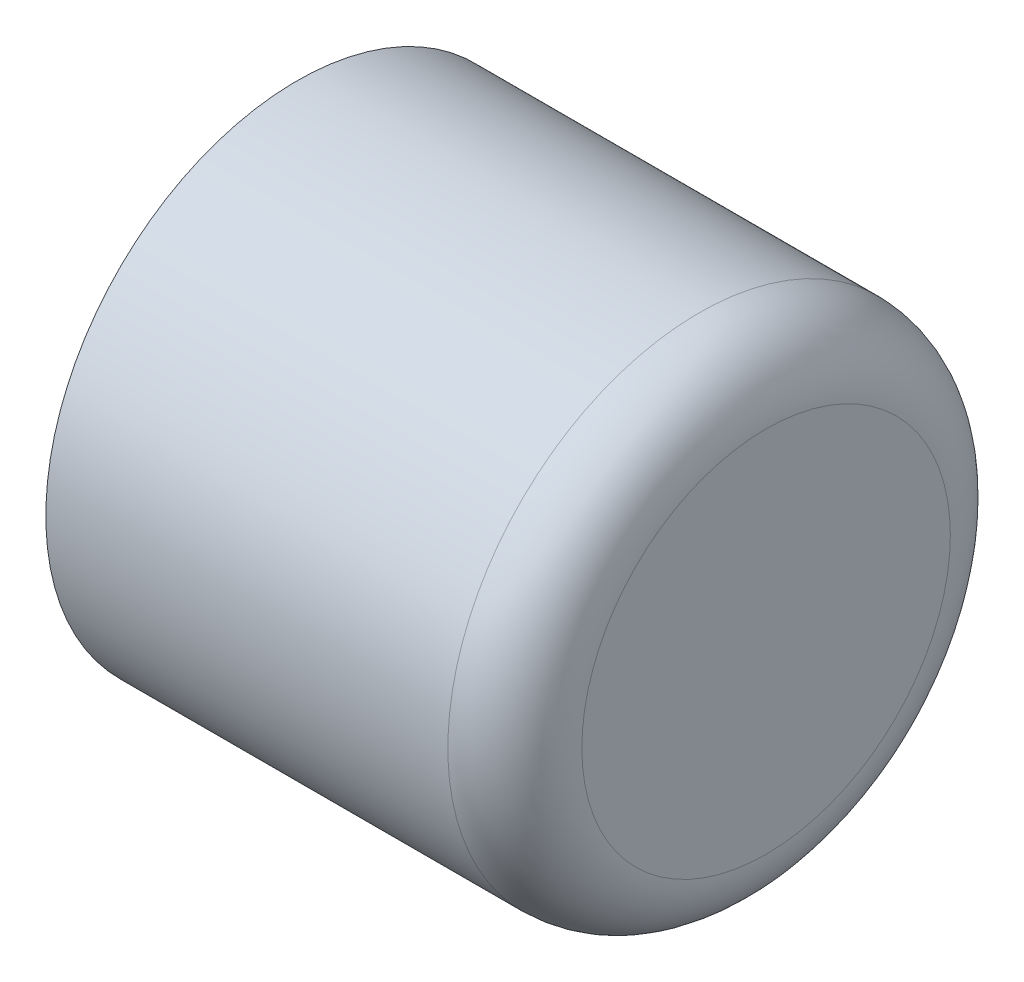
from build123d import *


with BuildPart() as part:
    # Sketch1 → Revolve1 (revolve)
    with BuildSketch(Plane.XY, mode=Mode.PRIVATE) as revolve1_sk:
        with BuildLine():
            Line((0, 0), (0, 5.5))
            ThreePointArc((0, 5.5), (-0.585786438, 6.914213562), (-2, 7.5))
            Line((-2, 7.5), (-14, 7.5))
            Line((-14, 7.5), (-14, 4))
            Line((-14, 4), (-2.017114914, 4))
            Line((-2.017114914, 4), (-2.017114914, 0))
            Line((-2.017114914, 0), (0, 0))
        make_face()
    revolve(revolve1_sk.sketch.rotate(Axis((0, 0, 0), (-1, 0, 0)), 90), axis=Axis((0, 0, 0), (-1, 0, 0)))


solid = part.part
